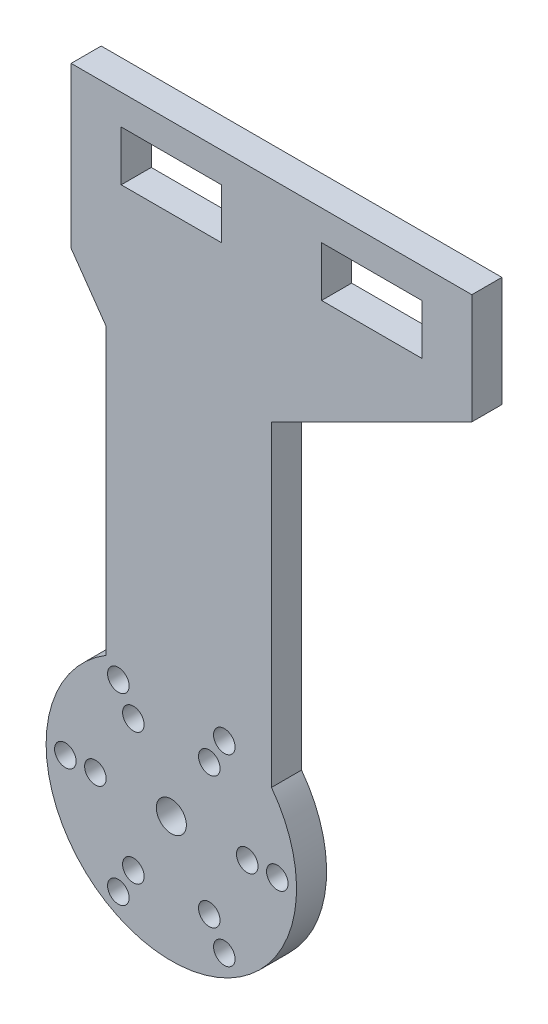
SolidWorks part; units mm, degrees
ref_plane "前视基准面" through (0, 0, 0) normal (0, 0, 1) x (1, 0, 0)
ref_plane "上视基准面" through (0, 0, 0) normal (0, 1, 0) x (1, 0, 0)
ref_plane "右视基准面" through (0, 0, 0) normal (1, 0, 0) x (0, 0, -1)
other "Configuration Table"
sketch "草图1" plane through (0, 0, 0) normal (0, 0, 1) x (1, 0, 0)
  line L0 (-78.5668, 0) -> (99.4491, 0) construction
  line L1 (0, 60.7924) -> (0, -59.8527) construction
  line L2 (-15.405, -13.3343) -> (-15.405, 15.0901)
  line L3 (-15.405, 15.0901) -> (-18.905, 20.0887)
  line L4 (-18.905, 20.0887) -> (-18.905, 36.0887)
  line L5 (-18.905, 36.0887) -> (21.095, 36.0887)
  line L6 (21.095, 36.0887) -> (21.095, 25.0887)
  line L7 (21.095, 25.0887) -> (1.095, 15.0887)
  line L8 (1.095, 15.0887) -> (1.095, -16.5113)
  line L9 (-13.905, 28.0887) -> (-3.905, 28.0887)
  line L10 (-13.905, 28.0887) -> (-13.905, 33.0887)
  line L11 (-13.905, 33.0887) -> (-3.905, 33.0887)
  line L12 (-3.905, 28.0887) -> (-3.905, 33.0887)
  line L13 (6.095, 28.0887) -> (16.095, 28.0887)
  line L14 (6.095, 28.0887) -> (6.095, 33.0887)
  line L15 (6.095, 33.0887) -> (16.095, 33.0887)
  line L16 (16.095, 28.0887) -> (16.095, 33.0887)
  arc A0 (-15.405, -13.3343) -> (1.095, -16.5113) centre (-8.905, -24.0113) ccw
  circle A1 centre (-8.905, -24.0113) radius 1.5
  circle A2 centre (-1.325, -24.0113) radius 1.075
  circle A3 centre (1.675, -24.0113) radius 1.075
  circle A4 centre (-5.115, -30.5758) radius 1.075
  circle A5 centre (-3.615, -33.1739) radius 1.075
  circle A6 centre (-12.695, -30.5758) radius 1.075
  circle A7 centre (-14.195, -33.1739) radius 1.075
  circle A8 centre (-16.485, -24.0113) radius 1.075
  circle A9 centre (-19.485, -24.0113) radius 1.075
  circle A10 centre (-12.695, -17.4469) radius 1.075
  circle A11 centre (-14.195, -14.8488) radius 1.075
  circle A12 centre (-5.115, -17.4469) radius 1.075
  circle A13 centre (-3.615, -14.8488) radius 1.075
  point P20 (6.095, 30.5887)
  dimension "D1" = 12.5
  dimension "D14" = 3
  dimension "D16" = 2.15
  dimension "D2" = 60.1
  dimension "D3" = 35
  dimension "D4" = 16
  dimension "D5" = 40
  dimension "D6" = 31.6
  dimension "D7" = 11
  dimension "D8" = 10
  dimension "D9" = 5
  dimension "D10" = 5
  dimension "D11" = 10
  dimension "D12" = 3
  dimension "D13" = 3
  dimension "D15" = 3
extrude "凸台-拉伸1" add sketch "草图1" along normal blind 3
